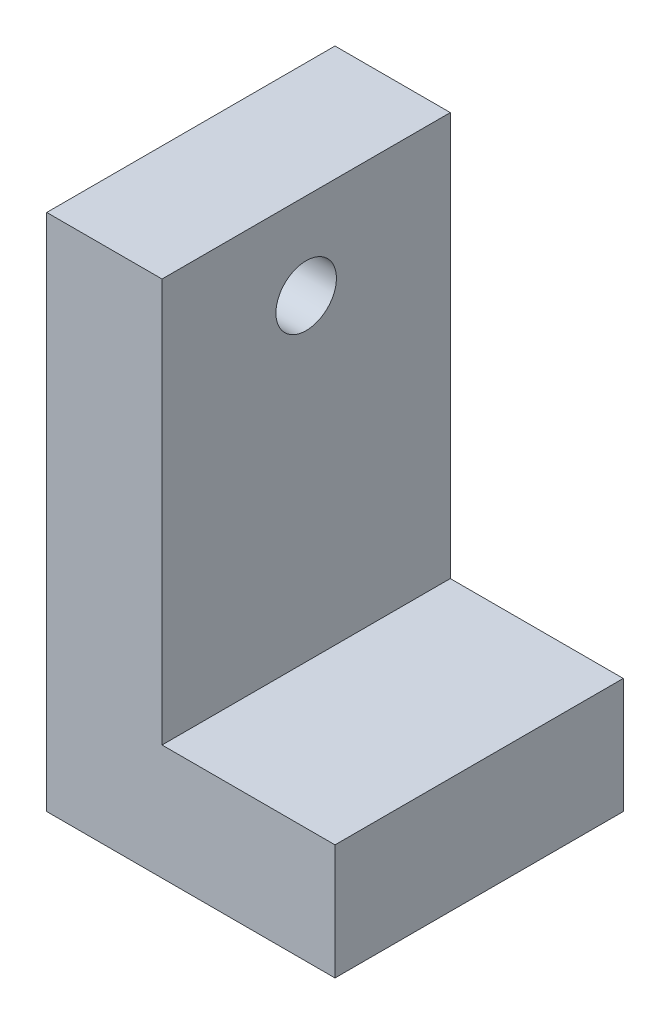
SolidWorks part; units mm, degrees
ref_plane "前视基准面" through (0, 0, 0) normal (0, 0, 1) x (1, 0, 0)
ref_plane "上视基准面" through (0, 0, 0) normal (0, 1, 0) x (1, 0, 0)
ref_plane "右视基准面" through (0, 0, 0) normal (1, 0, 0) x (0, 0, -1)
sketch "草图1" plane through (0, 0, 0) normal (0, 0, 1) x (1, 0, 0)
  line L0 (0, 0) -> (-20, 0)
  line L1 (-20, 0) -> (-20, 36)
  line L2 (-20, 36) -> (-12, 36)
  line L3 (-12, 36) -> (-12, 8)
  line L4 (-12, 8) -> (0, 8)
  line L5 (0, 8) -> (0, 0)
  dimension "D1" = 12
  dimension "D2" = 8
  dimension "D3" = 28
  dimension "D4" = 8
extrude "凸台-拉伸1" add sketch "草图1" along normal mid plane 20
hole_wizard "M5 螺纹孔1" positions "3D草图1" profile "草图3" tap size "M5" standard "GB" end condition up to next
sketch3d "3D草图1"
  line L0 (-20, 30, 0) -> (-20, 36, 0)
  line L1 (-20, 36, 10) -> (-20, 36, -10) construction
  point P0 (-20, 30, 0)
  dimension "D1" = 6
sketch "草图3" plane through (-20, 30, 0) normal (0, 1, 0) x (0, 0, 1)
  line L0 (0, 0) -> (0, 8)
  line L1 (0, 8) -> (2.1, 8)
  line L2 (2.1, 8) -> (2.1, 0)
  line L5 (2.1, 0) -> (0, 0)
  line L11 (0, -6.35) -> (0, 107.95) construction
  dimension "通孔螺纹孔钻头直径" = 4.2
  dimension "通孔螺纹孔钻头深度" = 8
